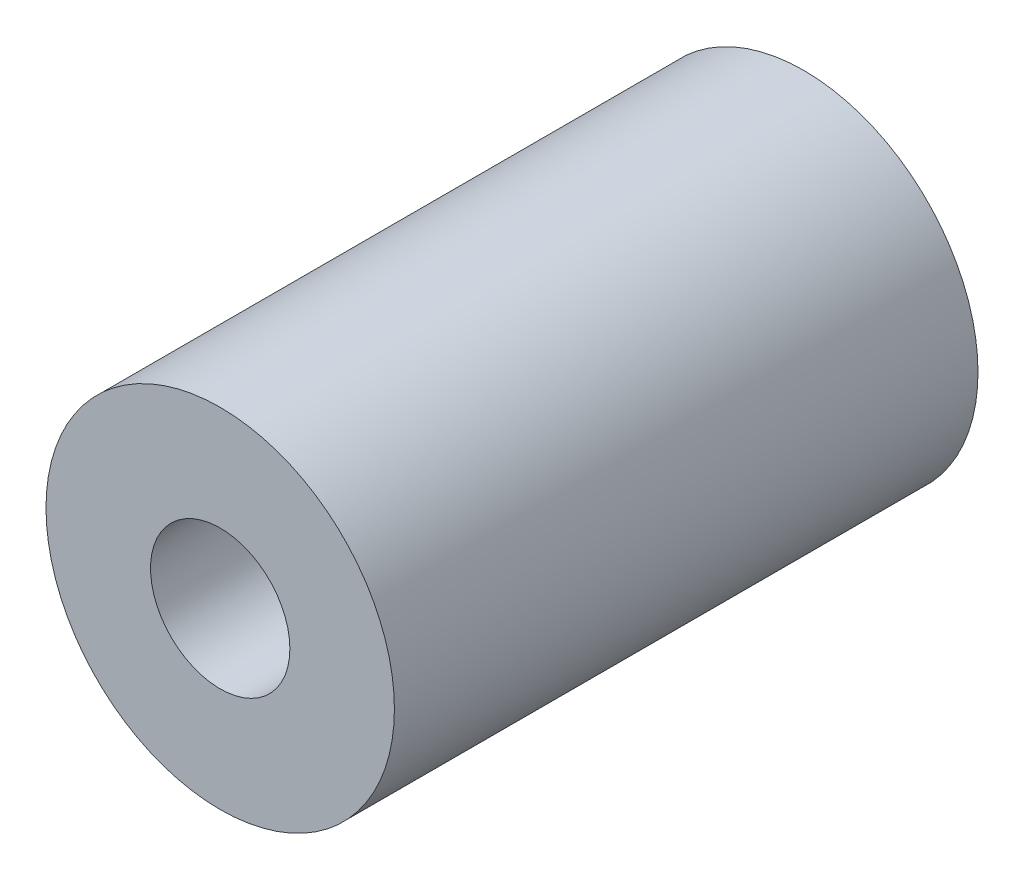
from build123d import *

# Parameters (mm, degrees)
SKETCH_1_R          = 20
EXTRUDE_1_DEPTH     = 67
SKETCH_2_R          = 8
CUT_EXTRUDE_1_DEPTH = 101


with BuildPart() as part:
    # 草图1 → 凸台-拉伸1 (new body)
    with BuildSketch(Plane.XY):
        Circle(SKETCH_1_R)
    extrude(amount=EXTRUDE_1_DEPTH)

    # 草图2 → 切除-拉伸1 (cut)
    with BuildSketch(Plane.XY.offset(67)):
        Circle(SKETCH_2_R)
    extrude(amount=-CUT_EXTRUDE_1_DEPTH, mode=Mode.SUBTRACT)


solid = part.part
